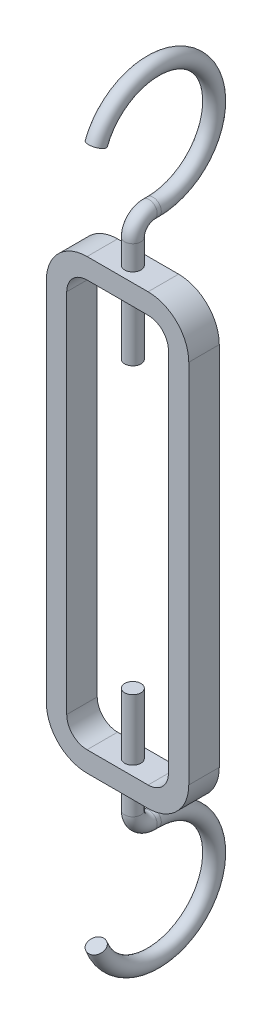
SolidWorks part; units mm, degrees
ref_plane "前视基准面" through (0, 0, 0) normal (0, 0, 1) x (1, 0, 0)
ref_plane "上视基准面" through (0, 0, 0) normal (0, 1, 0) x (1, 0, 0)
ref_plane "右视基准面" through (0, 0, 0) normal (1, 0, 0) x (0, 0, -1)
other "Configuration Table"
sketch "草图1" [suppressed] plane through (0, 0, 0) normal (0, 0, 1) x (1, 0, 0)
  line L0 (-1429.5042, 682.106) -> (-1603.2354, 423.5)
  line L2 (-1595.571, 405.0268) -> (-1610.8998, 441.9731)
  point P5 (-1603.2354, 423.5)
sketch "草图2" [suppressed] plane through (0, 0, 0) normal (0, 0, 1) x (1, 0, 0)
  line L0 (-1429.5042, 682.106) -> (-1603.2354, 423.5) construction
  line L1 (-1429.5042, 682.106) -> (-1603.2354, 423.5)
sketch "草图4" plane through (0, 0, 0) normal (0, 0, 1) x (1, 0, 0)
  line L0 (-15, 110) -> (15, 110)
  line L1 (-15, -100) -> (15, -100)
  line L2 (-25, -90) -> (-25, 90)
  line L3 (-15, 100) -> (15, 100)
  line L4 (25, -90) -> (25, 90)
  line L5 (-25, -100) -> (25, 100) construction
  line L6 (-25, 100) -> (25, -100) construction
  line L7 (35, -90) -> (35, 90)
  line L8 (-15, -110) -> (15, -110)
  line L9 (-35, -90) -> (-35, 90)
  arc A0 (15, -100) -> (25, -90) centre (15, -90) ccw
  arc A1 (-25, 90) -> (-15, 100) centre (-15, 90) cw
  arc A2 (-15, -100) -> (-25, -90) centre (-15, -90) cw
  arc A3 (15, 100) -> (25, 90) centre (15, 90) cw
  arc A4 (15, 110) -> (35, 90) centre (15, 90) cw
  arc A5 (15, -110) -> (35, -90) centre (15, -90) ccw
  arc A6 (-15, -110) -> (-35, -90) centre (-15, -90) cw
  arc A7 (-35, 90) -> (-15, 110) centre (-15, 90) cw
  point P0 (0, 0)
  dimension "D3" = 10
  dimension "D1" = 50
  dimension "D2" = 200
  dimension "D4" = 10
extrude "凸台-拉伸1" add sketch "草图4" along normal mid plane 15
sketch "草图5" plane through (0, 0, 0) normal (1, 0, 0) x (0, 0, -1)
  line L0 (0, 110) -> (0, 122)
  line L1 (-7.5, 110) -> (7.5, 110) construction
  line L2 (8, 130) -> (10, 130)
  arc A0 (10, 130) -> (-18, 170.7703) centre (10, 160) ccw
  arc A1 (0, 122) -> (8, 130) centre (8, 122) cw
  point P10 (0, 130)
  point P11 (0, 0)
  point P12 (0, 185.0432)
  point P13 (0, 0)
  point P14 (0, 0)
  point P15 (-18.9003, 168.048)
  dimension "D2" = 8
  dimension "D4" = 30
  dimension "D1" = 10
  dimension "D3" = 50
  dimension "D5" = 28
sketch "草图6" plane through (0, 110, 0) normal (0, 1, 0) x (1, 0, 0)
  circle A0 centre (0, 0) radius 4
  dimension "D1" = 8
sweep "扫描1" add profiles "草图6" path "草图5"
sketch "草图7" plane through (0, 100, 0) normal (0, -1, 0) x (1, 0, 0)
  circle A0 centre (0, 0) radius 4 construction
  circle A1 centre (0, 0) radius 4
extrude "凸台-拉伸2" add sketch "草图7" along normal blind 30 contours A1
mirror "镜向1" about plane through (0, 0, 0) normal (0, 1, 0) of "扫描1", "凸台-拉伸2"
